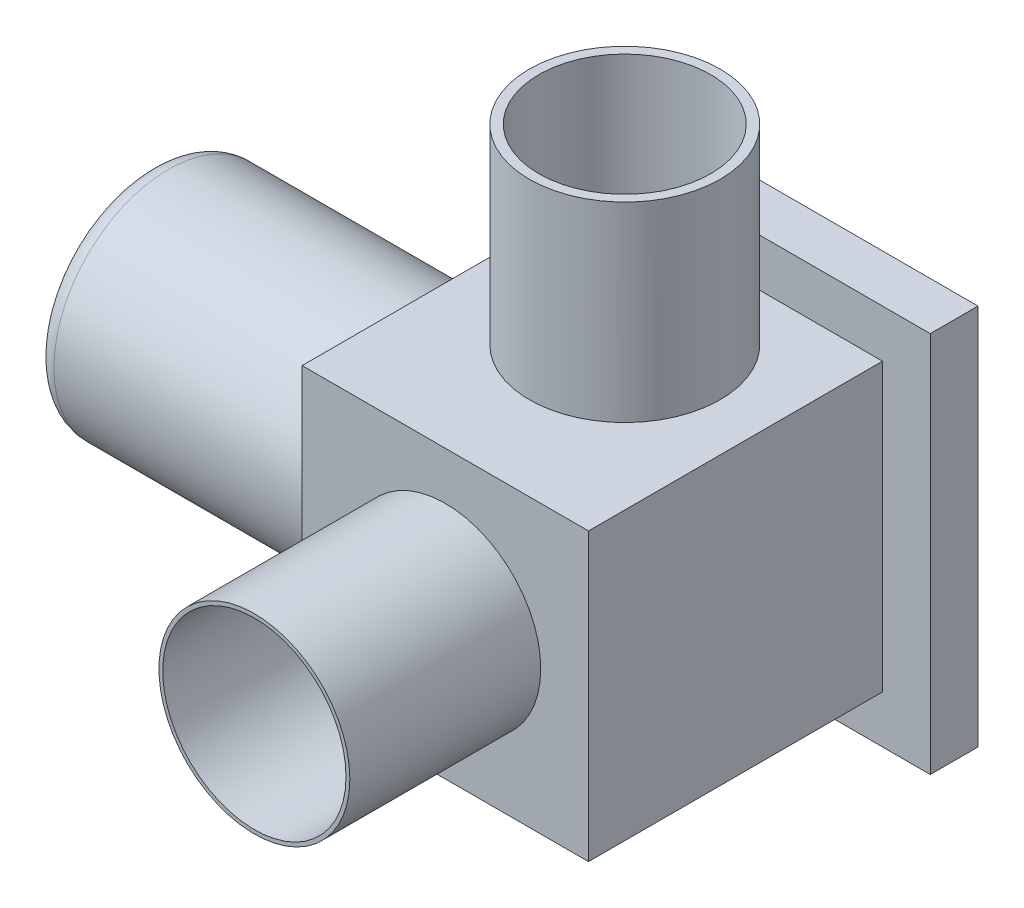
SolidWorks part; units mm, degrees
ref_plane "前视基准面" through (0, 0, 0) normal (0, 0, 1) x (1, 0, 0)
ref_plane "上视基准面" through (0, 0, 0) normal (0, 1, 0) x (1, 0, 0)
ref_plane "右视基准面" through (0, 0, 0) normal (1, 0, 0) x (0, 0, -1)
sketch "草图1" plane through (0, 0, 0) normal (0, 0, 1) x (1, 0, 0)
  line L1 (-100, -100) -> (100, -100)
  line L2 (-100, -100) -> (-100, 100)
  line L3 (-100, 100) -> (100, 100)
  line L4 (100, -100) -> (100, 100)
  line L5 (-100, -100) -> (100, 100) construction
  line L6 (-100, 100) -> (100, -100) construction
  point P0 (0, 0)
  dimension "D1" = 200
  dimension "D2" = 200
extrude "凸台-拉伸1" add sketch "草图1" along normal blind 25
sketch "草图2" plane through (0, 0, 25) normal (0, 0, 1) x (1, 0, 0)
  line L1 (-75, -75) -> (75, -75)
  line L2 (-75, -75) -> (-75, 75)
  line L3 (-75, 75) -> (75, 75)
  line L4 (75, -75) -> (75, 75)
  line L5 (-75, -75) -> (75, 75) construction
  line L6 (-75, 75) -> (75, -75) construction
  point P0 (0, 0)
  dimension "D1" = 150
  dimension "D2" = 150
extrude "凸台-拉伸2" add sketch "草图2" along normal blind 154
sketch "草图3" plane through (-75, 0, 0) normal (1, 0, 0) x (0, 0, -1)
  line L0 (-25, -100) -> (-25, 100) construction
  line L1 (-179, -75) -> (-25, -75) construction
  circle A0 centre (-105, -5) radius 60
  dimension "D1" = 120
  dimension "D2" = 80
  dimension "D3" = 70
extrude "凸台-拉伸3" add sketch "草图3" against normal blind 154
fillet "圆角1" radius 10 1 edges at (-229, -5, 45)
sketch "草图4" plane through (0, 0, 179) normal (0, 0, 1) x (1, 0, 0)
  circle A0 centre (0, 0) radius 50
  dimension "D1" = 100
extrude "凸台-拉伸4" add sketch "草图4" along normal blind 100
sketch "草图5" plane through (0, 75, 0) normal (0, 1, 0) x (1, 0, 0)
  line L0 (0, 0) -> (0, -171.9924) construction
  line L1 (100, 0) -> (-100, 0) construction
  circle A0 centre (0, -85) radius 50
  circle A1 centre (0, -85) radius 45
  dimension "D1" = 100
  dimension "D2" = 85
  dimension "D3" = 90
extrude "凸台-拉伸5" add sketch "草图5" along normal blind 100
sketch "草图6" plane through (0, 0, 279) normal (0, 0, 1) x (1, 0, 0)
  circle A0 centre (0, 0) radius 48
  circle A1 centre (0, 0) radius 50 construction
  dimension "D1" = 2
extrude "切除-拉伸1" cut sketch "草图6" against normal up to surface (100 mm away) up to face at (50, 0, 179)
